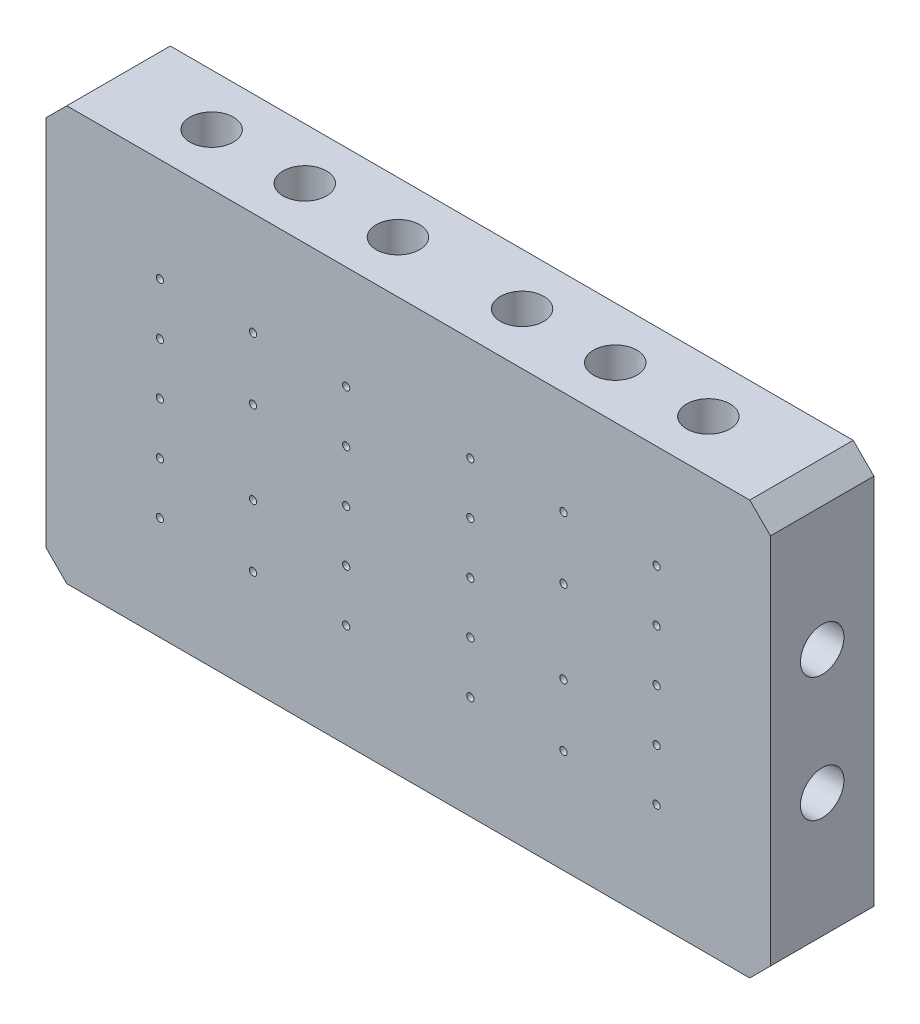
from build123d import *

# Parameters (mm, degrees)
SKETCH_1_W                        = 70
SKETCH_1_H                        = 40
EXTRUDE_1_DEPTH                   = 10
HOLE_WIZARD_3_2_3_2_1_D           = 3.2
HOLE_WIZARD_M5_1_D                = 4.2
HOLE_WIZARD_M5_1_DEPTH            = 11
HOLE_WIZARD_M5_1_TIP              = 1.2618073
HOLE_WIZARD_M5_2_D                = 4.2
HOLE_WIZARD_M5_2_DEPTH            = 12
HOLE_WIZARD_M5_2_TIP              = 1.2618073
HOLE_WIZARD_3_2_3_2_2_D           = 3.2
HOLE_WIZARD_3_2_3_2_2_DEPTH       = 46
HOLE_WIZARD_3_2_3_2_2_TIP         = 0.96137699
HOLE_WIZARD_0_7_0_7_2_AT_2_COUNT  = 2
HOLE_WIZARD_0_7_0_7_2_AT_2_PITCH  = 31.622776602
HOLE_WIZARD_0_7_0_7_2_AT_3_COUNT  = 2
HOLE_WIZARD_0_7_0_7_2_AT_3_PITCH  = 33.541019662
HOLE_WIZARD_0_7_0_7_2_AT_4_COUNT  = 2
HOLE_WIZARD_0_7_0_7_2_AT_4_PITCH  = 36.055512755
HOLE_WIZARD_0_7_0_7_2_AT_5_COUNT  = 2
HOLE_WIZARD_0_7_0_7_2_AT_5_PITCH  = 30
HOLE_WIZARD_0_7_0_7_2_AT_6_COUNT  = 2
HOLE_WIZARD_0_7_0_7_2_AT_6_PITCH  = 30.413812651
HOLE_WIZARD_0_7_0_7_2_AT_7_COUNT  = 2
HOLE_WIZARD_0_7_0_7_2_AT_7_PITCH  = 20
HOLE_WIZARD_0_7_0_7_2_AT_8_COUNT  = 2
HOLE_WIZARD_0_7_0_7_2_AT_8_PITCH  = 15
HOLE_WIZARD_0_7_0_7_2_AT_9_COUNT  = 2
HOLE_WIZARD_0_7_0_7_2_AT_9_PITCH  = 10
HOLE_WIZARD_0_7_0_7_2_AT_10_COUNT = 2
HOLE_WIZARD_0_7_0_7_2_AT_10_PITCH = 5
HOLE_WIZARD_0_7_0_7_3_AT_2_COUNT  = 2
HOLE_WIZARD_0_7_0_7_3_AT_2_PITCH  = 6
HOLE_WIZARD_0_7_0_7_3_AT_3_COUNT  = 2
HOLE_WIZARD_0_7_0_7_3_AT_3_PITCH  = 14
HOLE_WIZARD_0_7_0_7_3_AT_4_COUNT  = 2
HOLE_WIZARD_0_7_0_7_3_AT_4_PITCH  = 20
PATTERN_LINEAR_3_COUNT            = 2
PATTERN_LINEAR_3_PITCH            = 18
PATTERN_LINEAR_4_COUNT            = 2
PATTERN_LINEAR_4_PITCH            = 30
HOLE_WIZARD_M3_2_D                = 2.5
HOLE_WIZARD_M3_2_DEPTH            = 7.5
HOLE_WIZARD_M3_2_TIP              = 0.751075774
CHAMFER_1_SIZE                    = 2
HOLE_WIZARD_M5_4_D                = 4.2
HOLE_WIZARD_M5_4_DEPTH            = 12
HOLE_WIZARD_M5_4_TIP              = 1.2618073


with BuildPart() as part:
    # 草图1 → 凸台-拉伸1 (new body)
    with BuildSketch(Plane.XY):
        Rectangle(SKETCH_1_W, SKETCH_1_H)
    extrude(amount=EXTRUDE_1_DEPTH)

    # Ø3.2 (3.2) 直径孔1 (through all)
    with Locations(Plane(origin=(35, 0, 0), x_dir=(0, 0, -1), z_dir=(1, 0, 0))):
        with Locations((-5, 6), (-5, -6)):
            Hole(HOLE_WIZARD_3_2_3_2_1_D / 2)

    # M5 螺纹孔1
    with Locations(Plane(origin=(35, 0, 0), x_dir=(0, 0, -1), z_dir=(1, 0, 0))):
        with Locations((-5, -6), (-5, 6)):
            Hole(HOLE_WIZARD_M5_1_D / 2, depth=HOLE_WIZARD_M5_1_DEPTH)
            with Locations((0, 0, -(HOLE_WIZARD_M5_1_DEPTH + HOLE_WIZARD_M5_1_TIP / 2))):  # 118° drill point
                Cone(0, HOLE_WIZARD_M5_1_D / 2, HOLE_WIZARD_M5_1_TIP, mode=Mode.SUBTRACT)

    # M5 螺纹孔2
    with Locations(Plane.ZY.offset(35)):
        with Locations((5, 6), (5, -6)):
            Hole(HOLE_WIZARD_M5_2_D / 2, depth=HOLE_WIZARD_M5_2_DEPTH)
            with Locations((0, 0, -(HOLE_WIZARD_M5_2_DEPTH + HOLE_WIZARD_M5_2_TIP / 2))):  # 118° drill point
                Cone(0, HOLE_WIZARD_M5_2_D / 2, HOLE_WIZARD_M5_2_TIP, mode=Mode.SUBTRACT)

    # Ø3.2 (3.2) 直径孔2
    with Locations(Plane(origin=(0, 20, 0), x_dir=(1, 0, 0), z_dir=(0, 1, 0))):
        with Locations((-24, -5), (-15, -5), (-6, -5), (6, -5), (15, -5), (24, -5)):
            Hole(HOLE_WIZARD_3_2_3_2_2_D / 2, depth=HOLE_WIZARD_3_2_3_2_2_DEPTH)
            with Locations((0, 0, -(HOLE_WIZARD_3_2_3_2_2_DEPTH + HOLE_WIZARD_3_2_3_2_2_TIP / 2))):  # 118° drill point
                Cone(0, HOLE_WIZARD_3_2_3_2_2_D / 2, HOLE_WIZARD_3_2_3_2_2_TIP, mode=Mode.SUBTRACT)

    # 草图12 → Ø0.7 (0.7) 直径孔2 (revolve, cut)
    with BuildSketch(Plane(origin=(6, -10, 10), x_dir=(0, -1, 0), z_dir=(1, 0, 0))):
        Polygon((0, 0), (0, 5.210301217), (0.35, 5), (0.35, 0), align=None)
    hole_wizard_0_7_0_7_2 = revolve(axis=Axis((6, -10, 16.35), (0, 0, -1)), mode=Mode.SUBTRACT)

    # Ø0.7 (0.7) 直径孔2 at 2: Ø0.7 (0.7) 直径孔2 ×2
    with Locations(*[Vector(-0.9486832980505138, 0.316227766016838, 0) * (i * HOLE_WIZARD_0_7_0_7_2_AT_2_PITCH) for i in range(1, HOLE_WIZARD_0_7_0_7_2_AT_2_COUNT)]):
        add(hole_wizard_0_7_0_7_2, mode=Mode.SUBTRACT)

    # Ø0.7 (0.7) 直径孔2 at 3: Ø0.7 (0.7) 直径孔2 ×2
    with Locations(*[Vector(-0.894427190999916, 0.4472135954999581, 0) * (i * HOLE_WIZARD_0_7_0_7_2_AT_3_PITCH) for i in range(1, HOLE_WIZARD_0_7_0_7_2_AT_3_COUNT)]):
        add(hole_wizard_0_7_0_7_2, mode=Mode.SUBTRACT)

    # Ø0.7 (0.7) 直径孔2 at 4: Ø0.7 (0.7) 直径孔2 ×2
    with Locations(*[Vector(-0.8320502943378437, 0.5547001962252293, 0) * (i * HOLE_WIZARD_0_7_0_7_2_AT_4_PITCH) for i in range(1, HOLE_WIZARD_0_7_0_7_2_AT_4_COUNT)]):
        add(hole_wizard_0_7_0_7_2, mode=Mode.SUBTRACT)

    # Ø0.7 (0.7) 直径孔2 at 5: Ø0.7 (0.7) 直径孔2 ×2
    with Locations(*[(-i * HOLE_WIZARD_0_7_0_7_2_AT_5_PITCH, 0, 0) for i in range(1, HOLE_WIZARD_0_7_0_7_2_AT_5_COUNT)]):
        add(hole_wizard_0_7_0_7_2, mode=Mode.SUBTRACT)

    # Ø0.7 (0.7) 直径孔2 at 6: Ø0.7 (0.7) 直径孔2 ×2
    with Locations(*[Vector(-0.9863939238321437, 0.16439898730535737, 0) * (i * HOLE_WIZARD_0_7_0_7_2_AT_6_PITCH) for i in range(1, HOLE_WIZARD_0_7_0_7_2_AT_6_COUNT)]):
        add(hole_wizard_0_7_0_7_2, mode=Mode.SUBTRACT)

    # Ø0.7 (0.7) 直径孔2 at 7: Ø0.7 (0.7) 直径孔2 ×2
    with Locations(*[(0, i * HOLE_WIZARD_0_7_0_7_2_AT_7_PITCH, 0) for i in range(1, HOLE_WIZARD_0_7_0_7_2_AT_7_COUNT)]):
        add(hole_wizard_0_7_0_7_2, mode=Mode.SUBTRACT)

    # Ø0.7 (0.7) 直径孔2 at 8: Ø0.7 (0.7) 直径孔2 ×2
    with Locations(*[(0, i * HOLE_WIZARD_0_7_0_7_2_AT_8_PITCH, 0) for i in range(1, HOLE_WIZARD_0_7_0_7_2_AT_8_COUNT)]):
        add(hole_wizard_0_7_0_7_2, mode=Mode.SUBTRACT)

    # Ø0.7 (0.7) 直径孔2 at 9: Ø0.7 (0.7) 直径孔2 ×2
    with Locations(*[(0, i * HOLE_WIZARD_0_7_0_7_2_AT_9_PITCH, 0) for i in range(1, HOLE_WIZARD_0_7_0_7_2_AT_9_COUNT)]):
        add(hole_wizard_0_7_0_7_2, mode=Mode.SUBTRACT)

    # Ø0.7 (0.7) 直径孔2 at 10: Ø0.7 (0.7) 直径孔2 ×2
    with Locations(*[(0, i * HOLE_WIZARD_0_7_0_7_2_AT_10_PITCH, 0) for i in range(1, HOLE_WIZARD_0_7_0_7_2_AT_10_COUNT)]):
        add(hole_wizard_0_7_0_7_2, mode=Mode.SUBTRACT)

    # 草图20 → Ø0.7 (0.7) 直径孔3 (revolve, cut)
    with BuildSketch(Plane(origin=(-15, 10, 10), x_dir=(0, -1, 0), z_dir=(1, 0, 0))):
        Polygon((0, 0), (0, 5.210301217), (0.35, 5), (0.35, 0), align=None)
    hole_wizard_0_7_0_7_3 = revolve(axis=Axis((-15, 10, 16.35), (0, 0, -1)), mode=Mode.SUBTRACT)

    # Ø0.7 (0.7) 直径孔3 at 2: Ø0.7 (0.7) 直径孔3 ×2
    with Locations(*[(0, -i * HOLE_WIZARD_0_7_0_7_3_AT_2_PITCH, 0) for i in range(1, HOLE_WIZARD_0_7_0_7_3_AT_2_COUNT)]):
        add(hole_wizard_0_7_0_7_3, mode=Mode.SUBTRACT)

    # Ø0.7 (0.7) 直径孔3 at 3: Ø0.7 (0.7) 直径孔3 ×2
    with Locations(*[(0, -i * HOLE_WIZARD_0_7_0_7_3_AT_3_PITCH, 0) for i in range(1, HOLE_WIZARD_0_7_0_7_3_AT_3_COUNT)]):
        add(hole_wizard_0_7_0_7_3, mode=Mode.SUBTRACT)

    # Ø0.7 (0.7) 直径孔3 at 4: Ø0.7 (0.7) 直径孔3 ×2
    with Locations(*[(0, -i * HOLE_WIZARD_0_7_0_7_3_AT_4_PITCH, 0) for i in range(1, HOLE_WIZARD_0_7_0_7_3_AT_4_COUNT)]):
        add(hole_wizard_0_7_0_7_3, mode=Mode.SUBTRACT)

    # 阵列(线性)3: Ø0.7 (0.7) 直径孔2 ×2
    with Locations(*[(i * PATTERN_LINEAR_3_PITCH, 0, 0) for i in range(1, PATTERN_LINEAR_3_COUNT)]):
        add(hole_wizard_0_7_0_7_2, mode=Mode.SUBTRACT)

    # 阵列(线性)3 copy 1 sketch → 阵列(线性)3 copy 1 (revolve, cut)
    with BuildSketch(Plane(origin=(-6, 0, 10), x_dir=(0, -1, 0), z_dir=(1, 0, 0))):
        Polygon((0, 0), (0, 5.210301217), (0.35, 5), (0.35, 0), align=None)
    revolve(axis=Axis((-6, 0, 16.35), (0, 0, -1)), mode=Mode.SUBTRACT)

    # 阵列(线性)3 copy 2 sketch → 阵列(线性)3 copy 2 (revolve, cut)
    with BuildSketch(Plane(origin=(-6, 5, 10), x_dir=(0, -1, 0), z_dir=(1, 0, 0))):
        Polygon((0, 0), (0, 5.210301217), (0.35, 5), (0.35, 0), align=None)
    revolve(axis=Axis((-6, 5, 16.35), (0, 0, -1)), mode=Mode.SUBTRACT)

    # 阵列(线性)3 copy 3 sketch → 阵列(线性)3 copy 3 (revolve, cut)
    with BuildSketch(Plane(origin=(-6, 10, 10), x_dir=(0, -1, 0), z_dir=(1, 0, 0))):
        Polygon((0, 0), (0, 5.210301217), (0.35, 5), (0.35, 0), align=None)
    revolve(axis=Axis((-6, 10, 16.35), (0, 0, -1)), mode=Mode.SUBTRACT)

    # 阵列(线性)3 copy 4 sketch → 阵列(线性)3 copy 4 (revolve, cut)
    with BuildSketch(Plane(origin=(-6, -10, 10), x_dir=(0, -1, 0), z_dir=(1, 0, 0))):
        Polygon((0, 0), (0, 5.210301217), (0.35, 5), (0.35, 0), align=None)
    revolve(axis=Axis((-6, -10, 16.35), (0, 0, -1)), mode=Mode.SUBTRACT)

    # 阵列(线性)3 copy 5 sketch → 阵列(线性)3 copy 5 (revolve, cut)
    with BuildSketch(Plane(origin=(-6, -5, 10), x_dir=(0, -1, 0), z_dir=(1, 0, 0))):
        Polygon((0, 0), (0, 5.210301217), (0.35, 5), (0.35, 0), align=None)
    revolve(axis=Axis((-6, -5, 16.35), (0, 0, -1)), mode=Mode.SUBTRACT)

    # 阵列(线性)3 copy 6 sketch → 阵列(线性)3 copy 6 (revolve, cut)
    with BuildSketch(Plane(origin=(24, 10, 10), x_dir=(0, -1, 0), z_dir=(1, 0, 0))):
        Polygon((0, 0), (0, 5.210301217), (0.35, 5), (0.35, 0), align=None)
    revolve(axis=Axis((24, 10, 16.35), (0, 0, -1)), mode=Mode.SUBTRACT)

    # 阵列(线性)3 copy 7 sketch → 阵列(线性)3 copy 7 (revolve, cut)
    with BuildSketch(Plane(origin=(24, 5, 10), x_dir=(0, -1, 0), z_dir=(1, 0, 0))):
        Polygon((0, 0), (0, 5.210301217), (0.35, 5), (0.35, 0), align=None)
    revolve(axis=Axis((24, 5, 16.35), (0, 0, -1)), mode=Mode.SUBTRACT)

    # 阵列(线性)3 copy 8 sketch → 阵列(线性)3 copy 8 (revolve, cut)
    with BuildSketch(Plane(origin=(24, 0, 10), x_dir=(0, -1, 0), z_dir=(1, 0, 0))):
        Polygon((0, 0), (0, 5.210301217), (0.35, 5), (0.35, 0), align=None)
    revolve(axis=Axis((24, 0, 16.35), (0, 0, -1)), mode=Mode.SUBTRACT)

    # 阵列(线性)3 copy 9 sketch → 阵列(线性)3 copy 9 (revolve, cut)
    with BuildSketch(Plane(origin=(24, -5, 10), x_dir=(0, -1, 0), z_dir=(1, 0, 0))):
        Polygon((0, 0), (0, 5.210301217), (0.35, 5), (0.35, 0), align=None)
    revolve(axis=Axis((24, -5, 16.35), (0, 0, -1)), mode=Mode.SUBTRACT)

    # 阵列(线性)4: Ø0.7 (0.7) 直径孔3 ×2
    with Locations(*[(i * PATTERN_LINEAR_4_PITCH, 0, 0) for i in range(1, PATTERN_LINEAR_4_COUNT)]):
        add(hole_wizard_0_7_0_7_3, mode=Mode.SUBTRACT)

    # 阵列(线性)4 copy 1 sketch → 阵列(线性)4 copy 1 (revolve, cut)
    with BuildSketch(Plane(origin=(15, 4, 10), x_dir=(0, -1, 0), z_dir=(1, 0, 0))):
        Polygon((0, 0), (0, 5.210301217), (0.35, 5), (0.35, 0), align=None)
    revolve(axis=Axis((15, 4, 16.35), (0, 0, -1)), mode=Mode.SUBTRACT)

    # 阵列(线性)4 copy 2 sketch → 阵列(线性)4 copy 2 (revolve, cut)
    with BuildSketch(Plane(origin=(15, -4, 10), x_dir=(0, -1, 0), z_dir=(1, 0, 0))):
        Polygon((0, 0), (0, 5.210301217), (0.35, 5), (0.35, 0), align=None)
    revolve(axis=Axis((15, -4, 16.35), (0, 0, -1)), mode=Mode.SUBTRACT)

    # 阵列(线性)4 copy 3 sketch → 阵列(线性)4 copy 3 (revolve, cut)
    with BuildSketch(Plane(origin=(15, -10, 10), x_dir=(0, -1, 0), z_dir=(1, 0, 0))):
        Polygon((0, 0), (0, 5.210301217), (0.35, 5), (0.35, 0), align=None)
    revolve(axis=Axis((15, -10, 16.35), (0, 0, -1)), mode=Mode.SUBTRACT)

    # M3 螺纹孔2
    with Locations(Plane(origin=(0, 0, 0), x_dir=(-1, 0, 0), z_dir=(0, 0, -1))):
        with Locations((-30, 15), (0, 15), (30, 15), (-30, -15), (0, -15), (30, -15)):
            Hole(HOLE_WIZARD_M3_2_D / 2, depth=HOLE_WIZARD_M3_2_DEPTH)
            with Locations((0, 0, -(HOLE_WIZARD_M3_2_DEPTH + HOLE_WIZARD_M3_2_TIP / 2))):  # 118° drill point
                Cone(0, HOLE_WIZARD_M3_2_D / 2, HOLE_WIZARD_M3_2_TIP, mode=Mode.SUBTRACT)

    # 倒角1
    chamfer_1_edges = [part.edges().sort_by_distance(p)[0] for p in [
        (35, -20, 5),
        (-35, -20, 5),
        (-35, 20, 5),
        (35, 20, 5),
    ]]
    chamfer(chamfer_1_edges, length=CHAMFER_1_SIZE)

    # M5 螺纹孔4
    with Locations(Plane(origin=(0, 20, 0), x_dir=(1, 0, 0), z_dir=(0, 1, 0))):
        with Locations((-24, -5), (-15, -5), (-6, -5), (6, -5), (15, -5), (24, -5)):
            Hole(HOLE_WIZARD_M5_4_D / 2, depth=HOLE_WIZARD_M5_4_DEPTH)
            with Locations((0, 0, -(HOLE_WIZARD_M5_4_DEPTH + HOLE_WIZARD_M5_4_TIP / 2))):  # 118° drill point
                Cone(0, HOLE_WIZARD_M5_4_D / 2, HOLE_WIZARD_M5_4_TIP, mode=Mode.SUBTRACT)


solid = part.part
